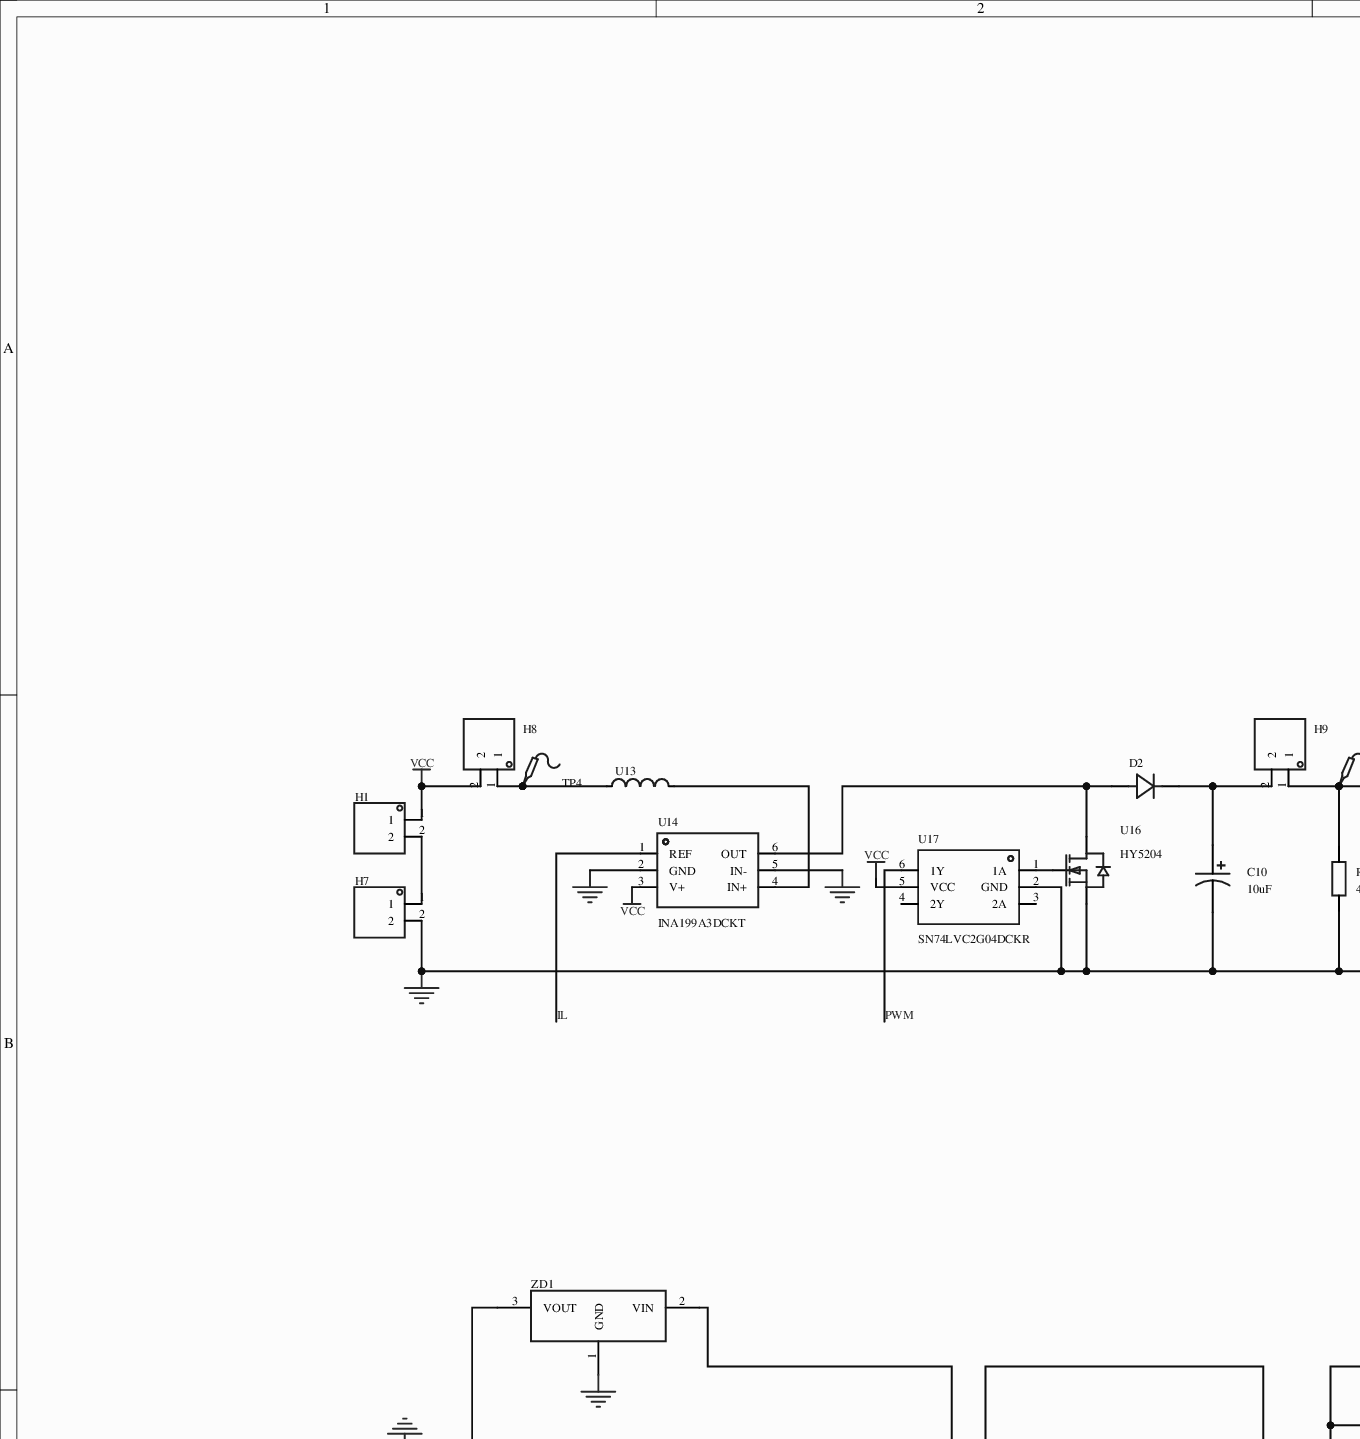
[diagram p0: MISC52076-3.schdoc, top left]
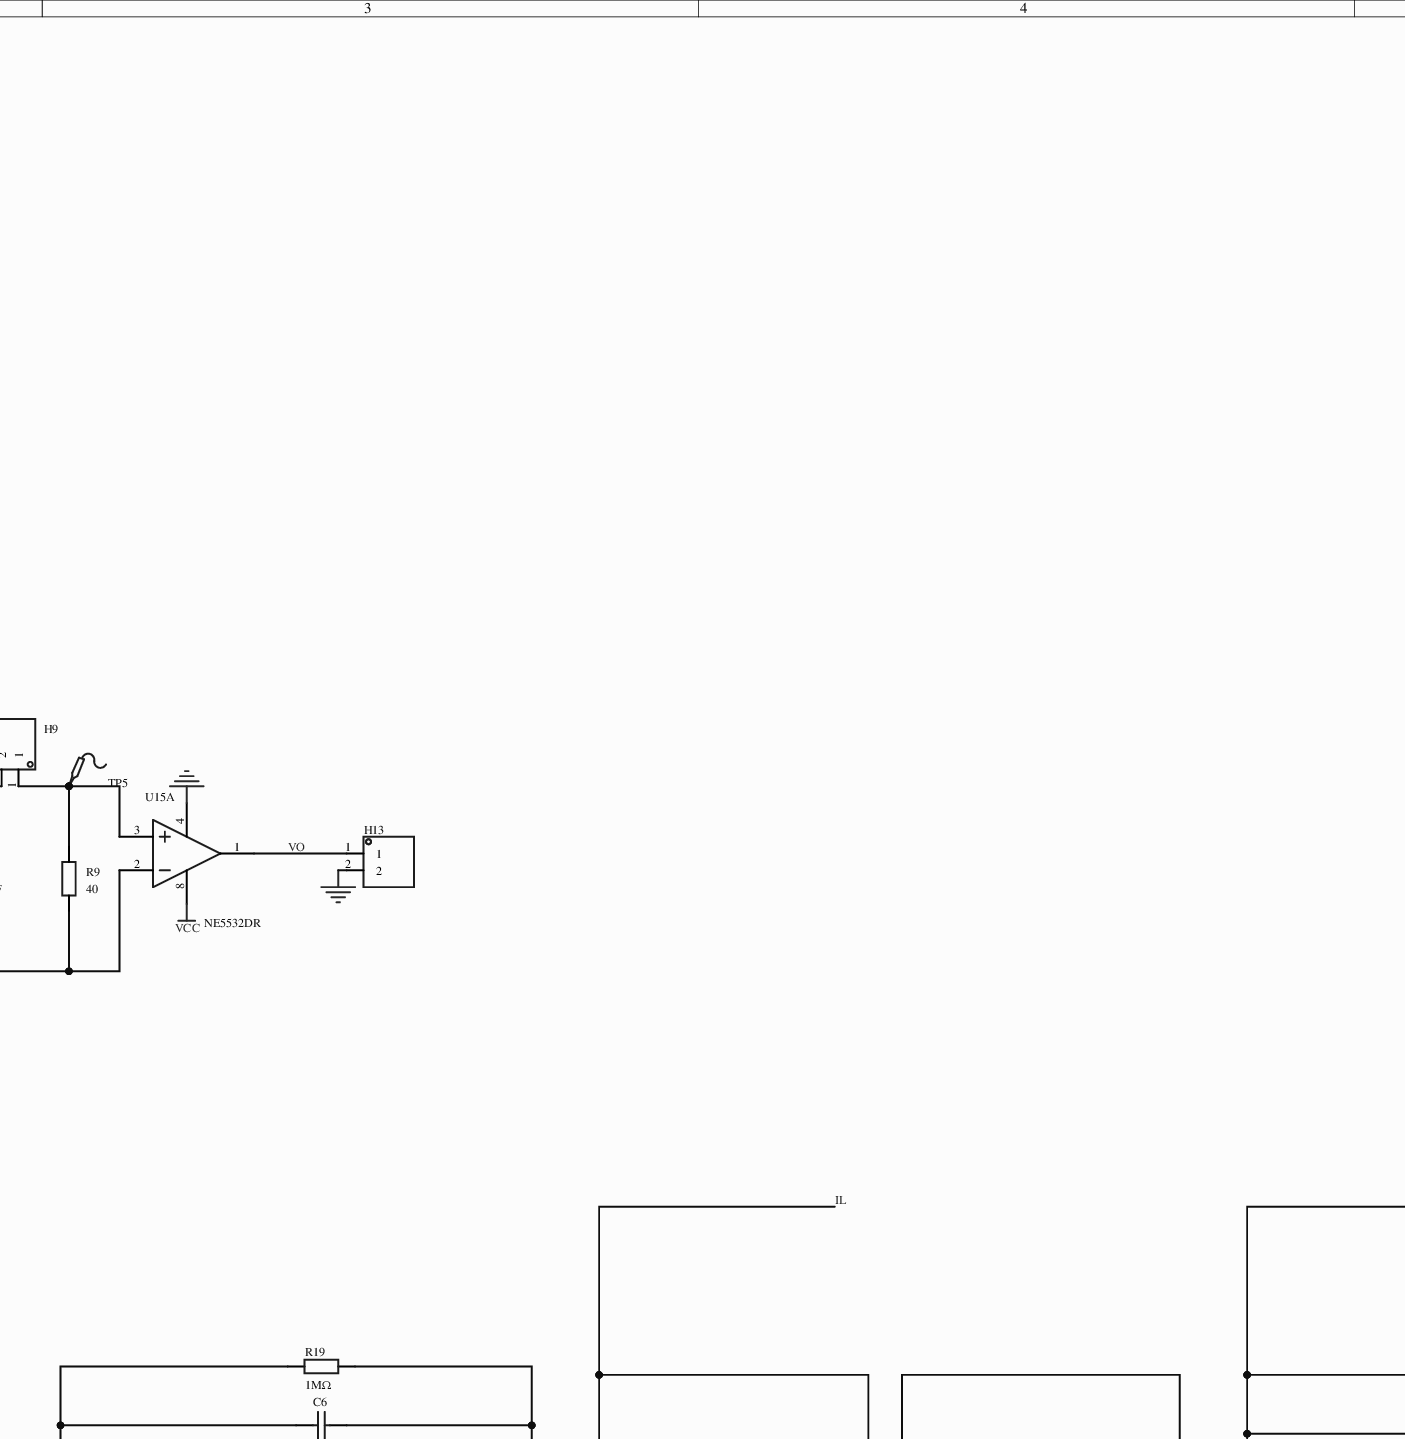
[diagram p1: MISC52076-3.schdoc, top middle]
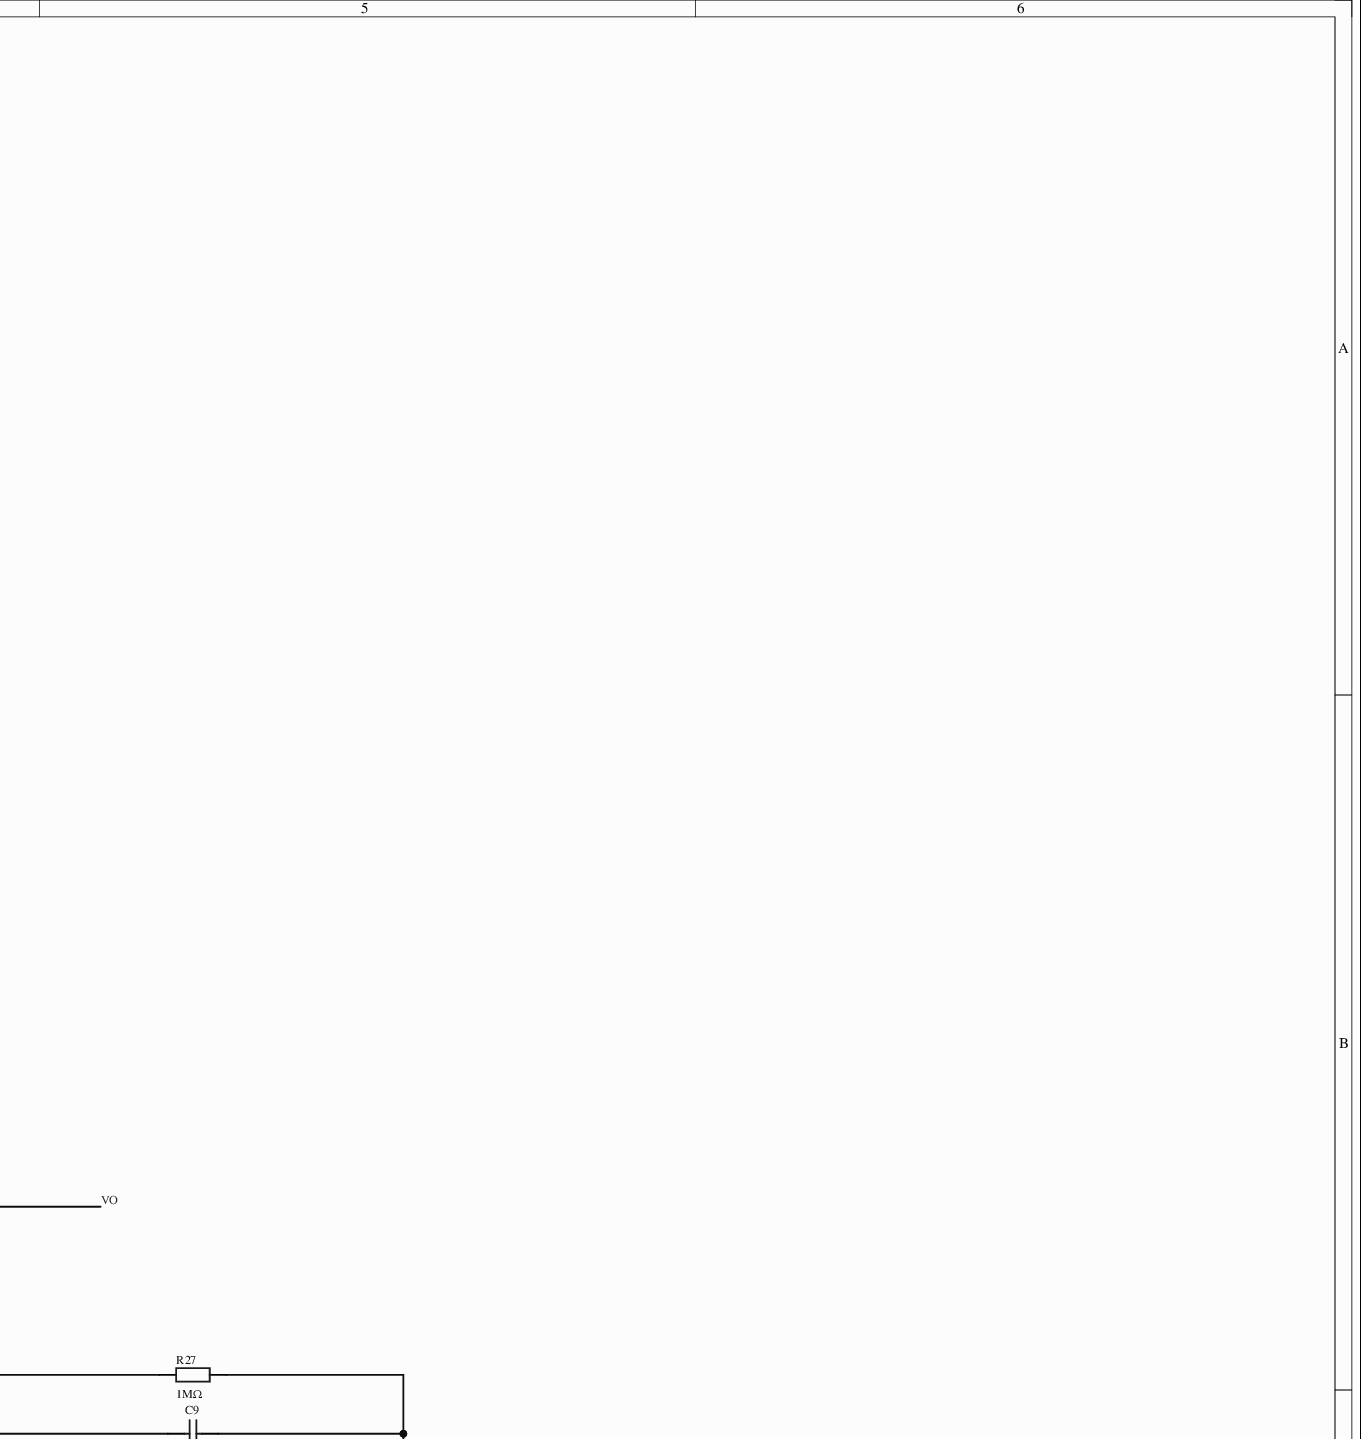
[diagram p2: MISC52076-3.schdoc, top right]
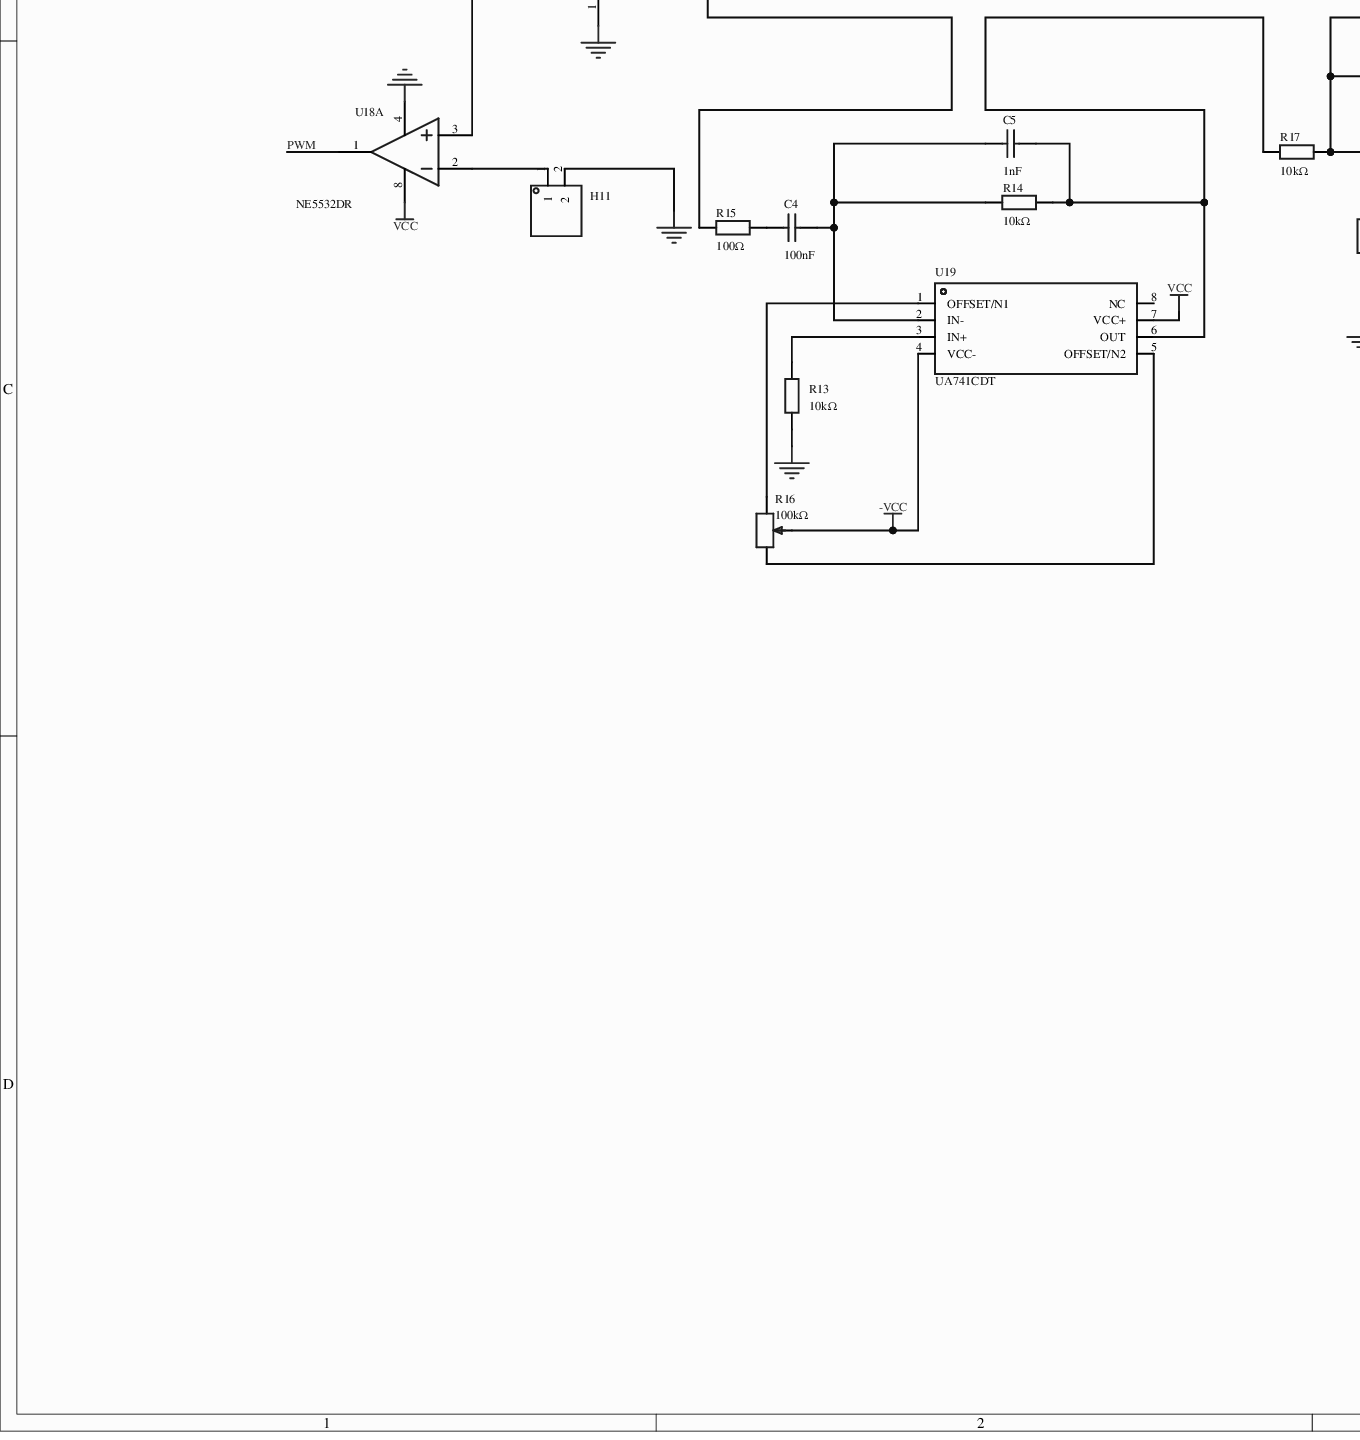
[diagram p3: MISC52076-3.schdoc, bottom left]
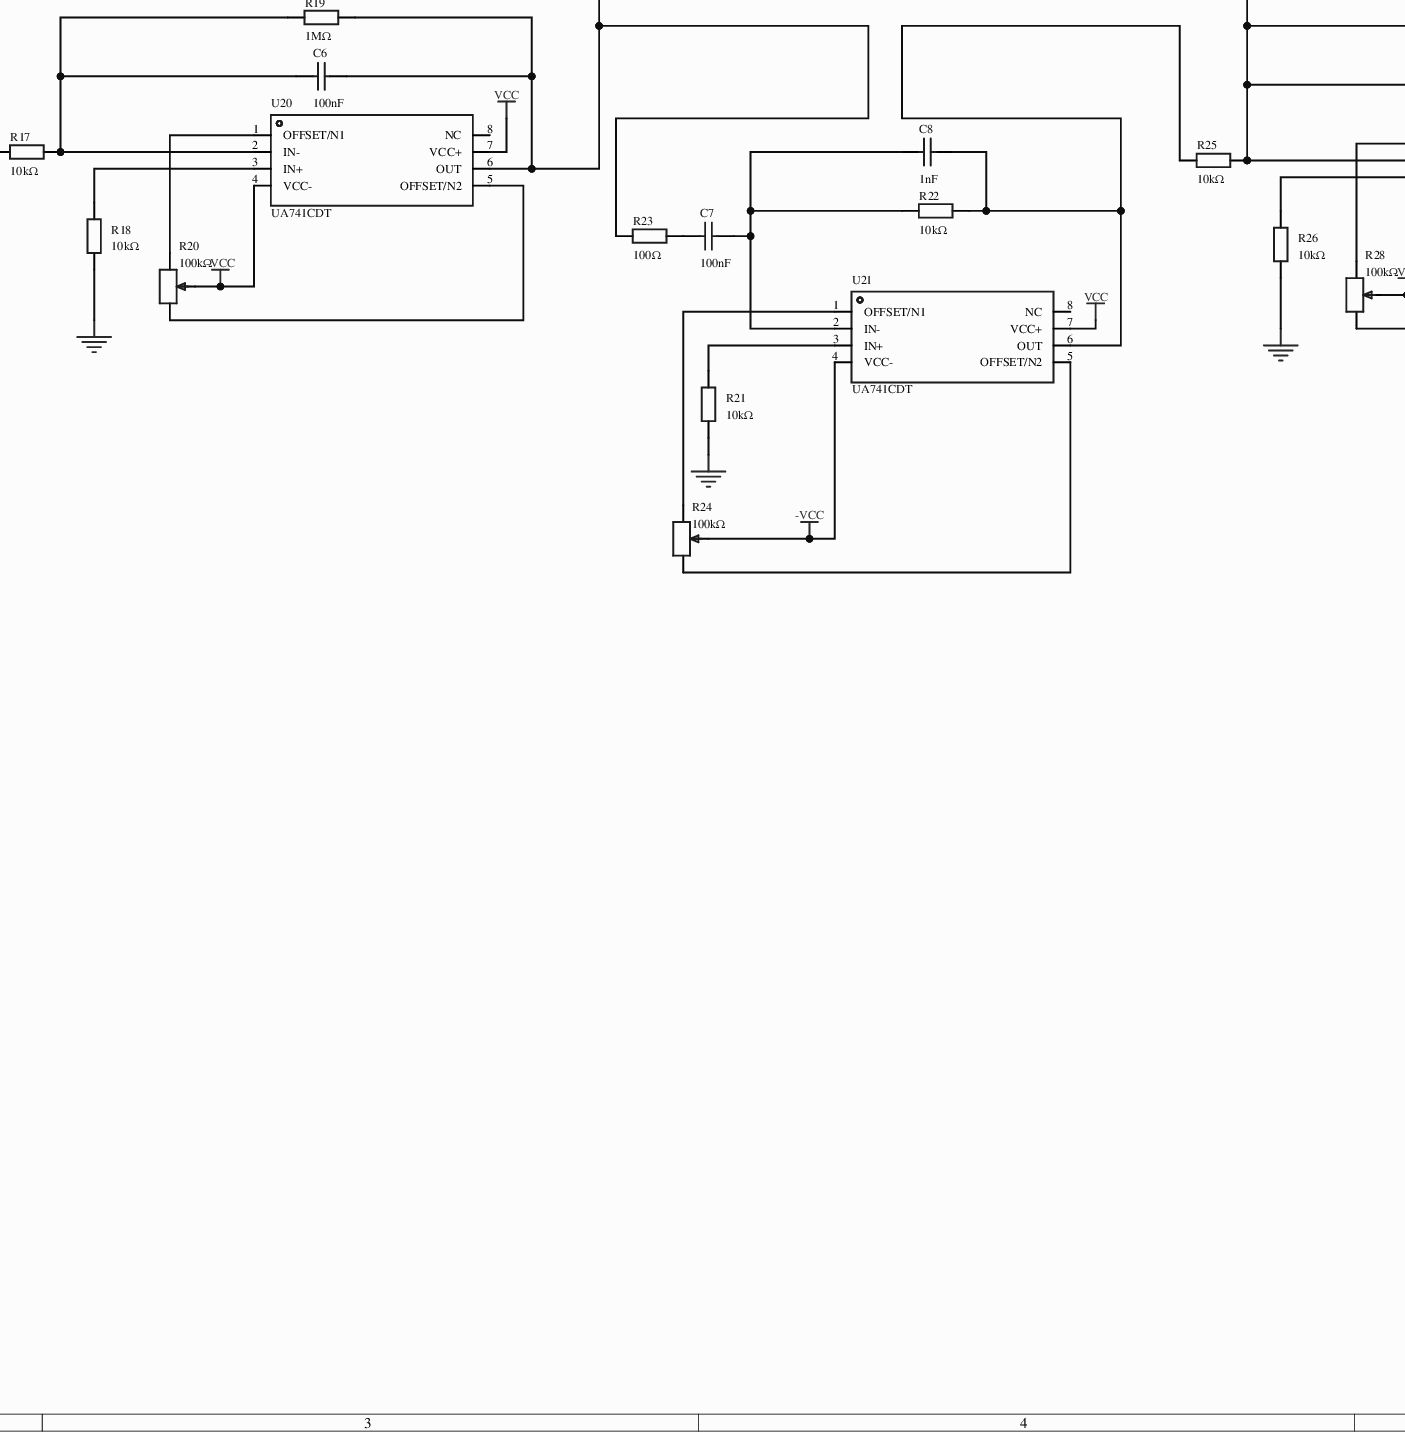
[diagram p4: MISC52076-3.schdoc, bottom middle]
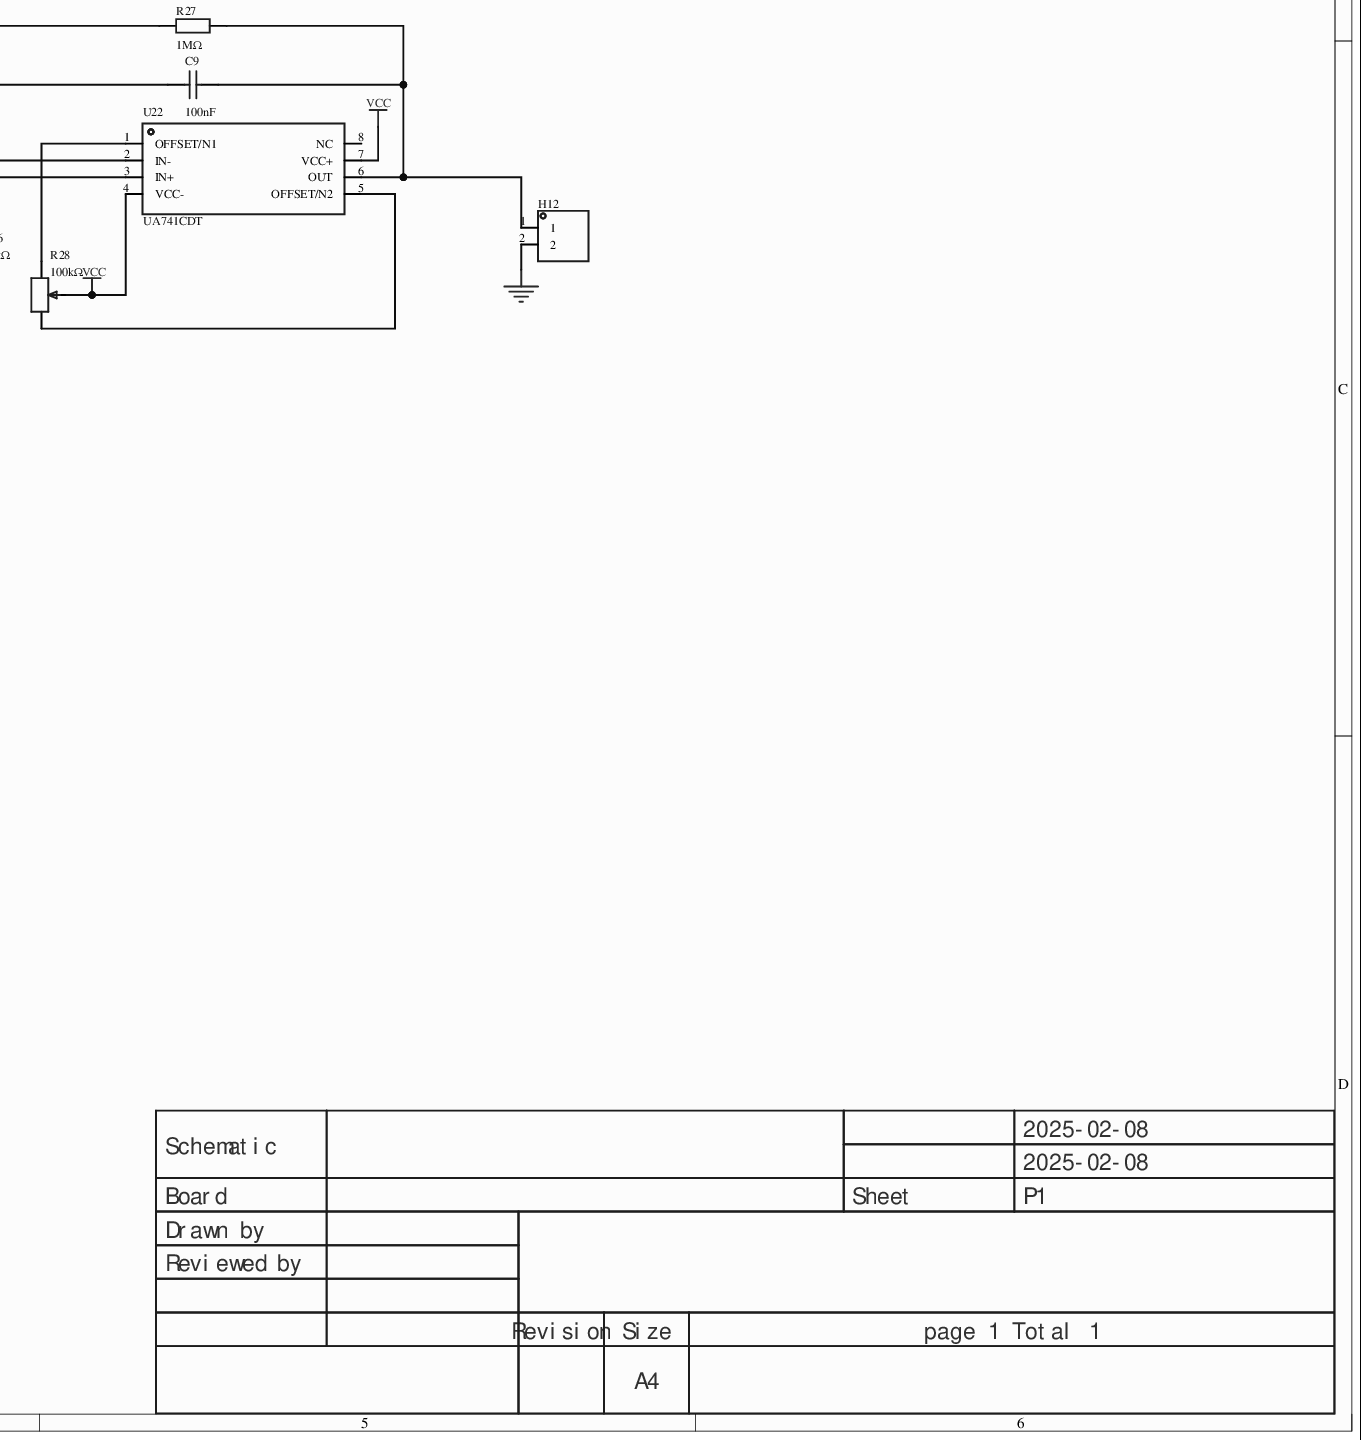
[diagram p5: MISC52076-3.schdoc, bottom right]
# Altium project MISC52076-2.PrjPcb
1 sheet, 45 parts. Net scope: global (net labels, ports and power ports of the same name join across sheets).
Board file: MISC52076.pcbdoc

## Sheet MISC52076-3.schdoc
size 594 x 419 mm; Version: V1.0; @Project Name: MISC52076; @Page Count: 1; @Update Date: 2025-02-08; @Create Date: 2025-02-08; @Schematic Name: MISC52076; @Page No: 1; @Create Time: 13:44:17; @Update Time: 13:44:25; @Board Name: MISC52076

### Parts
C4  100nF  [C0805]
C5  1nF  [C0805]
C6  100nF  [C0805]
C7  100nF  [C0805]
C8  1nF  [C0805]
C9  100nF  [C0805]
C10  10uF  [CAP-TH_BD4.0-P1.50-D0.8-FD]
D2  (no value)  [DO_1N4007]
H1  (no value)  [HDR-TH_2P-P2.54-V-M-1]
H7  (no value)  [HDR-TH_2P-P2.54-V-M-1]
H8  (no value)  [HDR-TH_2P-P2.54-V-M-1]
H9  (no value)  [HDR-TH_2P-P2.54-V-M-1]
H11  (no value)  [HDR-TH_2P-P2.54-V-M-1]
H12  (no value)  [HDR-TH_2P-P2.54-V-M-1]
H13  (no value)  [HDR-TH_2P-P2.54-V-M-1]
R9  40  [Res_1/4W]
R13  10kΩ  [R0805]
R14  10kΩ  [R0805]
R15  100Ω  [R0805]
R16  100kΩ  [RES-ADJ-SMD_VG039NCH]
R17  10kΩ  [R0805]
R18  10kΩ  [R0805]
R19  1MΩ  [R0805]
R20  100kΩ  [RES-ADJ-SMD_VG039NCH]
R21  10kΩ  [R0805]
R22  10kΩ  [R0805]
R23  100Ω  [R0805]
R24  100kΩ  [RES-ADJ-SMD_VG039NCH]
R25  10kΩ  [R0805]
R26  10kΩ  [R0805]
R27  1MΩ  [R0805]
R28  100kΩ  [RES-ADJ-SMD_VG039NCH]
TP4  (no value)  [Test-Point-0.5mm]
TP5  (no value)  [Test-Point-0.5mm]
U13  Power inductor (SMD), CKST0502-10uH/M, 10uH, ±20%, 3A, package 5.7mm*5.1mm*2.0mm, Cenke, RoHS  [IND-SMD_L5.7-W5.1]  (value not drawn)
U14  INA199A3DCKT  [SC-70-6_L2.1-W1.3-P0.65-LS2.1-BR]
U15  NE5532DR  [SOIC-8_L4.9-W3.9-P1.27-LS6.0-BL]  (part A of 2)
U16  HY5204  [TO-247-3_L15.8-W5.0-P5.44-L-1]
U17  SN74LVC2G04DCKR  [SOT-363_L2.0-W1.3-P0.65-LS2.1-BR]
U18  NE5532DR  [SOIC-8_L4.9-W3.9-P1.27-LS6.0-BL]  (part A of 2)
U19  UA741CDT  [SOIC-8_L4.9-W3.9-P1.27-LS6.0-BL]
U20  UA741CDT  [SOIC-8_L4.9-W3.9-P1.27-LS6.0-BL]
U21  UA741CDT  [SOIC-8_L4.9-W3.9-P1.27-LS6.0-BL]
U22  UA741CDT  [SOIC-8_L4.9-W3.9-P1.27-LS6.0-BL]
ZD1  (no value)  [SOT-89-3_L4.5-W2.5-P1.50-LS4.2-BR]

### Nets
-VCC: R16.2 R20.2 R24.2 R28.2 U19.4(VCC-) U20.4(VCC-) U21.4(VCC-) U22.4(VCC-)
GND: C10.2 H7.2 H11.2 H12.2 H13.2 R9.1 R13.1 R18.1 R21.1 R26.1 U14.2(GND) U14.5(IN-) U15.2(IN1-) U15.4(VCC-/GND) U16.3(S) U17.2(GND) U18.4(VCC-/GND) ZD1.1(GND)
VCC: H1.1 H8.2 U14.3(V+) U15.8(VCC+) U17.5(VCC) U18.8(VCC+) U19.7(VCC+) U20.7(VCC+) U21.7(VCC+) U22.7(VCC+)
IL: C6.2 R19.2 R23.1 U14.1(REF) U20.6(OUT)
PWM: U17.6(1Y) U18.1(OUT1)
VO: C9.1 H13.1 R25.2 R27.1 U15.1(OUT1) U22.2(IN-)
NetC4_1: C4.1 R15.2
NetC4_2: C4.2 C5.1 R14.1 U19.2(IN-)
NetC5_2: C5.2 R14.2 R17.1 U19.6(OUT)
NetC6_1: C6.1 R17.2 R19.1 U20.2(IN-)
NetC7_1: C7.1 R23.2
NetC7_2: C7.2 C8.1 R22.1 U21.2(IN-)
NetC8_2: C8.2 R22.2 R25.1 U21.6(OUT)
NetC9_2: C9.2 H12.1 R27.2 U22.6(OUT)
NetC10_1: C10.1 D2.1(K) H9.2
NetD2_2: D2.2(A) U14.6(OUT) U16.2(D)
NetH1_2: H1.2 H7.1
NetH8_1: H8.1 TP4.1 U13.1
NetH9_1: H9.1 R9.2 TP5.1 U15.3(IN1+)
NetH11_1: H11.1 U18.2(IN1-)
NetR13_2: R13.2 U19.3(IN+)
NetR15_1: R15.1 ZD1.2(VIN)
NetR16_1: R16.1 U19.1(OFFSET/N1)
NetR16_3: R16.3 U19.5(OFFSET/N2)
NetR18_2: R18.2 U20.3(IN+)
NetR20_1: R20.1 U20.5(OFFSET/N2)
NetR20_3: R20.3 U20.1(OFFSET/N1)
NetR21_2: R21.2 U21.3(IN+)
NetR24_1: R24.1 U21.1(OFFSET/N1)
NetR24_3: R24.3 U21.5(OFFSET/N2)
NetR26_2: R26.2 U22.3(IN+)
NetR28_1: R28.1 U22.5(OFFSET/N2)
NetR28_3: R28.3 U22.1(OFFSET/N1)
NetU13_2: U13.2 U14.4(IN+)
NetU16_1: U16.1(G) U17.1(1A)
NetU18_3: U18.3(IN1+) ZD1.3(VOUT)

Not connected (* = marked no-connect by the designer): U17 3(2A)* 4(2Y)*; U19 8(NC); U20 8(NC); U21 8(NC); U22 8(NC)

### Notes on the sheet
- 2025-02-08
- Schematic
- Board
- Sheet
- P1
- Drawn by
- Reviewed by
- Revision
- Size
- A4
- page 1 Total 1

### Library data of the parts
C4-C9 = CC0805KRX7R9BB104: Capacitance: 100nF; Tolerance: ±10%; Rated voltage: 50V; Dielectric (temperature coefficient): X7R;; Manufacturer: YAGEO(国巨); AddInBom: yes; ModelId: 1ba041120af144c991958decab20d241; ModelName: C0805_L2.0-W1.3-H1.3; ModelTransform: 78.74,51.181,0,0,0,0,0,0.0005,0; Symbol: CC0805KRX7R9BB104; Device: CC0805KRX7R9BB104; LCSC Part Name: 100nF ±10% 50V; ManufacturerPart: CC0805KRX7R9BB104; Supplier Footprint: 0805; JLCPCB Part Class: Basic library; Datasheet: https://atta.szlcsc.com/upload/public/pdf/source/20180224/C181747_15194369449651363981.pdf; Supplier: LCSC; ConvertToPcb: yes; FootprintName: C0805; Voltage Rated: 50V; Temperature Coefficient: X7R
  C4 C6 C7 C9: SupplierPart: C49678; Value: 100nF
  C5 C8: Value: 1nF
C10 = 10MS510MEFC4X5: Capacitance: 10uF; Tolerance: ±20%; Rated voltage: 10V; Ripple current: 16mA@120Hz;; Manufacturer: rubycon(红宝石); AddInBom: yes; ModelId: 8017ea3dd4884afab5fc61dd7898abc1; ModelName: CAP-TH_D4.0-H7.0-P1.5; ModelTransform: 158.2674,157.45008,0,0,0,0,0,0,-137.795; φD: 4mm; L: 5mm; Lifetime @ Temp: 1000hrs@85℃; Symbol: 10MS510MEFC4X5; Device: 10MS510MEFC4X5; LCSC Part Name: 10uF ±20% 10V; SupplierPart: C1579578; ManufacturerPart: 10MS510MEFC4X5; Supplier Footprint: 插件,D4xL5mm; JLCPCB Part Class: Extended library; Datasheet: https://atta.szlcsc.com/upload/public/pdf/source/20210510/C1579578_ABB61F9CFFB4E7371AD0DBD373B61F20.pdf; Supplier: LCSC; ConvertToPcb: yes; FootprintName: CAP-TH_BD4.0-P1.50-D0.8-FD; Value: 10uF; Rated Voltage: 10V; Ripple Current: 16mA@120Hz; Lead Spacing: 1.5mm; Operating Temperature: -40℃~+85℃
D2 = D_1N4007A: AddInBom: yes; ModelId: 6de1e9b71a0d4751b4e9df530304c1a3; ModelName: DO-41_D2.4-L4.7-P8.70; ModelTransform: 373.9,94.4,232.29,0,0,0,0,0,-140; Symbol: D_1N4007; Device: D_1N4007A; Supplier Footprint: DO-41; ConvertToPcb: yes; FootprintName: DO_1N4007
H1 H7-H9 H11-H13 = HDR-M_2.54_1x2P: Symbol: 210S-1*2P L=11.6MMGold-plated black; ConvertToPcb: yes; ModelId: 79b2e9f2d70a4d68a1b7098f27c6d4c5; ModelName: HDR-M-2.54_1x2; ModelTransform: 200,100,0,0,0,0,0,0,-118.11; Device: HDR-M_2.54_1x2P; AddInBom: yes; SupplierPart: C124375; Supplier Footprint: 插件; FootprintName: HDR-TH_2P-P2.54-V-M-1
R9 = Res_AXIAL-1/4W: AddInBom: yes; SymbolName: Resistor; ModelId: 463263665006444ab7a47bd11b0cf956; ModelName: RES-TH_BD2.4-L6.3-P10.30-D0.6; ModelTransform: 427.165,94.32816,0,0,0,0,0,0,-196.85; Value: 40; Device: Res_AXIAL-1/4W; Supplier Footprint: 轴向引线; ConvertToPcb: yes; FootprintName: Res_1/4W
R13-R15 R17-R19 R21-R23 R25-R27 = 0805W8F1002T5E_C17414: Resistor type: thick film resistor; Resistance: 10kΩ; Tolerance: ±1%; Power: 125mW; Max working voltage: 150V; Temperature coefficient: ±100ppm/℃;; Manufacturer: UNI-ROYAL(厚声); AddInBom: yes; ModelId: 37a81e68749a4138bd2dfa6897b24b85; ModelName: R0805_L2.0-W1.3-H0.6; ModelTransform: 78.74,51.181,0,0,0,0,0,-0.0005,0; Symbol: 0805W8F1002T5E; Device: 0805W8F1002T5E_C17414; Supplier: LCSC; Manufacturer Part: 0805W8F1002T5E; JLCPCB Part Class: Basic library; LCSC Part Name: 10kΩ ±1% 125mW 厚膜电阻; Supplier Footprint: 0805; Datasheet: https://atta.szlcsc.com/upload/public/pdf/source/20200306/C422600_1E6D84923E4A46A82E41ADD87F860B5C.pdf; ConvertToPcb: yes; FootprintName: R0805; Type: Thick film resistor; Power(Watts): 125mW; Overload Voltage (Max): 150V; Temperature Coefficient: ±100ppm/℃; Operating Temperature Range: -55℃~+155℃
  R13 R14 R17 R18 R21 R22 R25 R26: Supplier Part: C17414; Value: 10kΩ
  R15 R23: Value: 100Ω
  R19 R27: Value: 1MΩ
R16 R20 R24 R28 = VG039NCHXTB201: Resistance: 200Ω; Tolerance: ±25%;; Manufacturer: HDK(北陆电气); AddInBom: yes; ModelId: ba438d2707b74a9ab8400a10f68363a0; ModelName: RES-ADJ-SMD_3P-L3.8-W3.0-H1.2-P1.90; ModelTransform: 120.0785,161.61385,0,90,0,0,-3.74,-0.118,0; Value: 100kΩ; Device: VG039NCHXTB201; Symbol: VG039NCHXTB201; LCSC Part Name: 200Ω ±25%; ManufacturerPart: VG039NCHXTB201; Supplier Footprint: SMD; JLCPCB Part Class: Extended library; Datasheet: https://atta.szlcsc.com/upload/public/pdf/source/20171123/C145162_15114111014461137838.pdf; Supplier: LCSC; ConvertToPcb: yes; FootprintName: RES-ADJ-SMD_VG039NCH; Tolerance: ±25%
TP4 TP5 = Test-Point: Test Point; AddInBom: yes; Device: Test-Point; ConvertToPcb: yes; SymbolName: Test-Point; FootprintName: Test-Point-0.5mm
U13 = 功率电感(贴片),CKST0502-10uH/M,10uH,±20%,3A,封装5.7mm*5.1mm*2.0mm,岑科,RoHS: AddInBom: yes; ModelId: ffd856615f974dd9b1ff3f65e3b3100d; ModelTransform: 224.409,200.787,0,0,0,0,0,-0.591,0; Symbol: Power inductor (SMD), CKST0502-10UH/M, 10UH, ±20%, 3A, package 5.7MM*5.1MM*2.0MM, Cenke, ROHS; Device: Power inductor (SMD), CKST0502-10uH/M, 10uH, ±20%, 3A, package 5.7mm*5.1mm*2.0mm, Cenke, RoHS; LCSC Part Name: 功率电感(贴片),CKST0502-10uH/M,10uH,±20%,3A,封装5.7mm*5.1mm*2.0mm,岑科,RoHS; SupplierPart: C9900015114; ManufacturerPart: 功率电感(贴片),CKST0502-10uH/M,10uH,±20%,3A,封装5.7mm*5.1mm*2.0mm,岑科,RoHS; Supplier Footprint: 功率电感(贴片),CKST0502-10uH/M,10uH,±20%,3A,封装5.7mm*5.1mm*2.0mm,岑科,RoHS; JLCPCB Part Class: Extended library; Supplier: LCSC; ConvertToPcb: yes; FootprintName: IND-SMD_L5.7-W5.1; ModelName: IND-SMD_L5.7-W5.1
U14 = INA199A3DCKT: 26V bidirectional current sense amplifier 6-SC70 -40 to 125; Manufacturer: TI(德州仪器); AddInBom: yes; ModelId: df0ecfc958064819b5626ee1f8e5fd24; ModelTransform: 82.677,82.6,0,0,0,0,0,0,0; Supply Voltage: -300mV~26V; Supply Current: 88uA; Symbol: INA199A3DCKT; Device: INA199A3DCKT; LCSC Part Name: INA199A3DCKT; SupplierPart: C2155798; ManufacturerPart: INA199A3DCKT; Supplier Footprint: SC-70-6; JLCPCB Part Class: Extended library; Supplier: LCSC; ConvertToPcb: yes; FootprintName: SC-70-6_L2.1-W1.3-P0.65-LS2.1-BR; ModelName: SC-70-6_L2.1-W1.3-P0.65-LS2.1-BR; Operating Temperature: -40℃~+125℃
U15 U18 = NE5532DR: 放大器数:双路;增益带宽积(GBP):10MHz;输入偏置电流(Ib):200nA;压摆率(SR):9V/us;带宽(-3db):-;; Manufacturer: TI(德州仪器); Relevance: []; AddInBom: yes; ModelId: e81d2f7d937b4a6ab1dca543ff5d56a4; ModelName: SOIC-8_L4.9-W3.9-H1.7-LS6.0-P1.27; ModelTransform: 189.751,236.22,0,0,0,0,0.0005,0.0005,0; Number of Circuits: Dual; Gain Bandwidth Product(GBP): 10MHz; Current - Input Bias(Ib): 200nA; Slew Rate(SR): 9V/us; Output Current: 38mA; Supply Current: 8mA; Symbol: NE5532DR; Device: NE5532DR; LCSC Part Name: NE5532DR; SupplierPart: C7426; ManufacturerPart: NE5532DR; Supplier Footprint: SOIC-8; Supplier: LCSC; ConvertToPcb: yes; FootprintName: SOIC-8_L4.9-W3.9-P1.27-LS6.0-BL; -3db Bandwidth: -; Operating Temperature: 0℃~+70℃
U16 = HY5204: AddInBom: yes; ModelId: 27b35664da8045b09b6c38d0310660f0; ModelTransform: 614.17235,196.88937,0,0,0,0,0,7.874,-196.85; Symbol: HY5204; Device: HY5204; LCSC Part Name: HY5204; SupplierPart: C9900006698; ManufacturerPart: HY5204; Supplier Footprint: MOSFET-N; JLCPCB Part Class: Extended library; Supplier: LCSC; ConvertToPcb: yes; FootprintName: TO-247-3_L15.8-W5.0-P5.44-L-1; ModelName: TO-247-3_L15.8-W5.0-P5.44-L-1
U17 = SN74LVC2G04DCKR: Input type: -; Supply voltage: 1.65V~5.5V; Supply current (max): 10uA; Circuits: 2; Max propagation delay (tpd): 3.2ns@5V,50pF;; Manufacturer: TI(德州仪器); AddInBom: yes; ModelId: ea15c7b026c54341854a7f0d9614aed9; ModelName: SOT-363-6P_L2.0-W1.3-H1.1-LS2.0-P0.65; ModelTransform: 83.17133,78.74,0,180,0,0,0,0,0; Number of Circuits: 2; Sink Current: 32mA; High level range (VIH): 1.7V~2V; Low level range (VIL): 700mV~800mV; Symbol: SN74LVC2G04DCKR; Device: SN74LVC2G04DCKR; LCSC Part Name: 双路反相器; SupplierPart: C105251; ManufacturerPart: SN74LVC2G04DCKR; Supplier Footprint: SOT-363-6; JLCPCB Part Class: Extended library; Supplier: LCSC; ConvertToPcb: yes; FootprintName: SOT-363_L2.0-W1.3-P0.65-LS2.1-BR; Input Type: -; Supply Voltage(Single): 1.65V~5.5V; Supply Current (Max): 10uA; Number of Inputs: 2; Source Current: 32mA; Max Propagation Delay: 3.2ns@5V,50pF; Series: 74LVC series; Operating Temperature: -40℃~+125℃
U19-U22 = UA741CDT: 放大器数:单路;增益带宽积(GBP):1MHz;输入偏置电流(Ib):10nA;压摆率(SR):0.5V/us;带宽(-3db):-;; Manufacturer: ST(意法半导体); AddInBom: yes; ModelId: e81d2f7d937b4a6ab1dca543ff5d56a4; ModelName: SOIC-8_L4.9-W3.9-H1.7-LS6.0-P1.27; ModelTransform: 189.751,236.22,0,0,0,0,0.0005,0.0005,0; Number of Circuits: Single; Gain Bandwidth Product(GBP): 1MHz; Current - Input Bias(Ib): 10nA; Output Current: 25mA; Supply Current: 3.3mA; Symbol: UA741CDT; Device: UA741CDT; LCSC Part Name: UA741CDT; SupplierPart: C7111; ManufacturerPart: UA741CDT; Supplier Footprint: SOIC-8; JLCPCB Part Class: Extended library; Datasheet: https://atta.szlcsc.com/upload/public/pdf/source/20181030/C283333_E7CFD90DFDEB0B09152BEF9966FA2369.pdf; Supplier: LCSC; ConvertToPcb: yes; FootprintName: SOIC-8_L4.9-W3.9-P1.27-LS6.0-BL; Slew Rate(SR): 0.5V/us; -3db Bandwidth: -; Operating Temperature: 0℃~+70℃
ZD1 = HT7233SOT89三端稳压300MA3.3VLDO稳压器: AddInBom: yes; ModelId: 6db690b7897d4d18a30d90c1b89525ee; ModelName: SOT-89-3_L4.3-W2.5-H1.6-LS4.1-P1.50; ModelTransform: 161.417,169.291,0,180,0,0,-11.808,0,0; Symbol: HT7233SOT89三端稳压300MA3.3VLDO稳压器; Device: HT7233SOT89三端稳压300MA3.3VLDO稳压器; LCSC Part Name: HT7233SOT89三端稳压300MA3.3VLDO稳压器; SupplierPart: C9900016143; Supplier Footprint: SOT-89-3; JLCPCB Part Class: Extended library; Supplier: LCSC; ConvertToPcb: yes; FootprintName: SOT-89-3_L4.5-W2.5-P1.50-LS4.2-BR